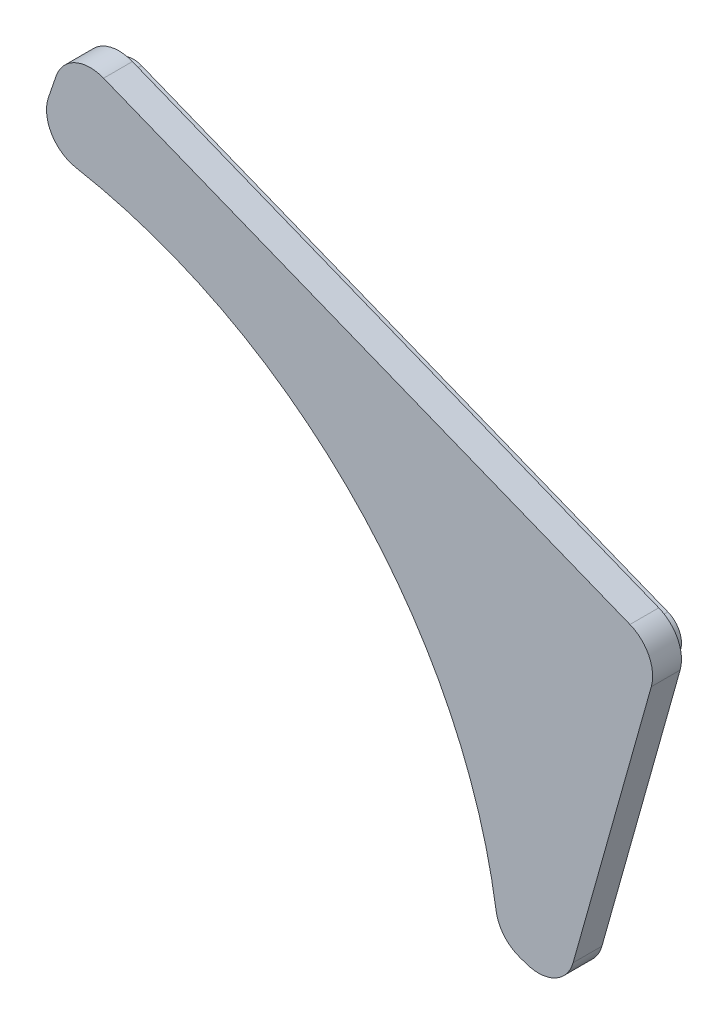
from build123d import *

# Parameters (mm, degrees)
EXTRUDE_1_DEPTH = 2
EXTRUDE_2_DEPTH = 4


with BuildPart() as part:
    # 草图1 → 凸台-拉伸1 (new body)
    with BuildSketch(Plane.XY):
        with BuildLine():
            Line((-151.259122885, 113.481956899), (-140.412267192, 152.068606889))
            ThreePointArc((-140.412267192, 152.068606889), (-140.610396656, 154.208706418), (-142.189143758, 155.667074982))
            Line((-142.189143758, 155.667074982), (-215.208108923, 184.78392473))
            ThreePointArc((-215.208108923, 184.78392473), (-217.571105228, 184.723649859), (-219.156952171, 182.97080244))
            Line((-219.156952171, 182.97080244), (-220.220905282, 179.86948426))
            ThreePointArc((-220.220905282, 179.86948426), (-219.971910037, 177.379794621), (-217.922197627, 175.944792124))
            ThreePointArc((-217.922197627, 175.944792124), (-178.080420962, 154.651932226), (-158.04090319, 114.165258148))
            ThreePointArc((-158.04090319, 114.165258148), (-157.378743964, 112.691016779), (-156.047834036, 111.774217336))
            Line((-156.047834036, 111.774217336), (-155.120685935, 111.456145455))
            ThreePointArc((-155.120685935, 111.456145455), (-152.753497975, 111.637181572), (-151.259122885, 113.481956899))
        make_face()
    extrude(amount=-EXTRUDE_1_DEPTH)

    # 草图2 → 凸台-拉伸2 (add)
    with BuildSketch(Plane.XY):
        with BuildLine():
            Line((-141.448352929, 157.524823337), (-214.467318094, 186.641673085))
            ThreePointArc((-214.467318094, 186.641673085), (-218.40564527, 186.541214966), (-221.048723508, 183.619802601))
            Line((-221.048723508, 183.619802601), (-222.112676618, 180.518484421))
            ThreePointArc((-222.112676618, 180.518484421), (-221.697684544, 176.369001689), (-218.281497194, 173.977330861))
            ThreePointArc((-218.281497194, 173.977330861), (-179.516525304, 153.259953663), (-160.01861612, 113.86751402))
            ThreePointArc((-160.01861612, 113.86751402), (-158.91501741, 111.410445071), (-156.696834197, 109.882445999))
            Line((-156.696834197, 109.882445999), (-155.769686096, 109.564374118))
            ThreePointArc((-155.769686096, 109.564374118), (-151.824372829, 109.86610098), (-149.33374768, 112.940726525))
            Line((-149.33374768, 112.940726525), (-138.486891987, 151.527376515))
            ThreePointArc((-138.486891987, 151.527376515), (-138.81710776, 155.094209064), (-141.448352929, 157.524823337))
        make_face()
    extrude(amount=EXTRUDE_2_DEPTH)


solid = part.part
